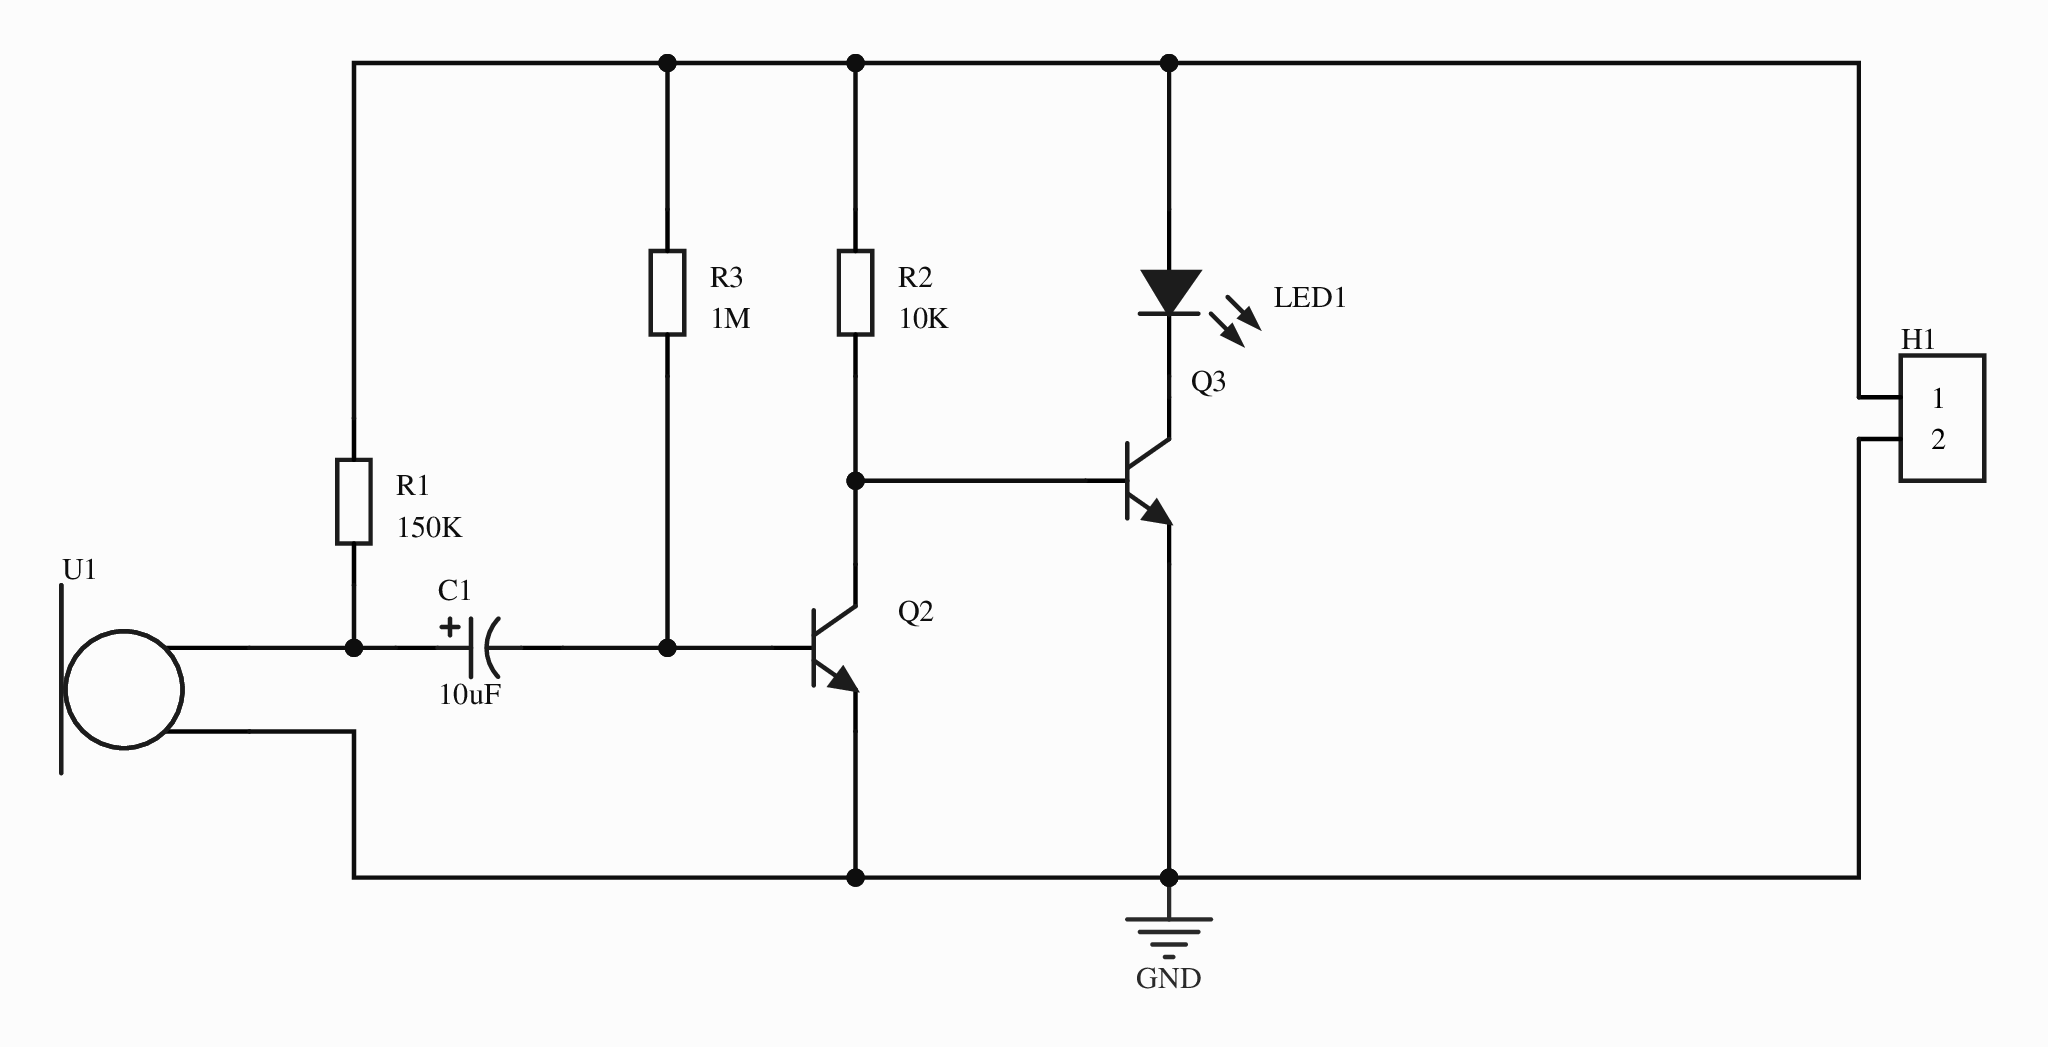
[diagram p0: MISC52075-3.schdoc]
# Altium project MISC52075-2.PrjPcb
1 sheet, 9 parts. Net scope: global (net labels, ports and power ports of the same name join across sheets).
Board file: MISC52075.pcbdoc

## Sheet MISC52075-3.schdoc
size 297 x 209 mm; Version: V1.0; @Project Name: MISC52075; @Update Date: 2026-10-05; @Create Date: 2026-10-05; @Board Name: MISC52075; @Create Time: 20:24:00; @Page Count: 1; @Page No: 1; @Schematic Name: MISC52075; @Update Time: 20:24:00; Size: A4

### Parts
C1  10uF  [CAP-TH_BD5.0-P2.00-D0.8-FD-10UF50VC110GL]
H1  (no value)  [HDR-TH_2P-P2.54-V-F]
LED1  (no value)  [LED_0603]
Q2  (no value)  [S8050_SOT-23]
Q3  (no value)  [S8050_SOT-23]
R1  150K  [R0603]
R2  10K  [R0603]
R3  1M  [R0603]
U1  电流源  [咪头]  (value not drawn)

### Nets
GND: H1.2 Q2.2 Q3.2 U1.1
NetC1_1: C1.1 R1.1 U1.2
NetC1_2: C1.2 Q2.1 R3.1
NetH1_1: H1.1 LED1.2(A) R1.2 R2.2 R3.2
NetLED1_1: LED1.1(C) Q3.3
NetQ2_3: Q2.3 Q3.1 R2.1

### Library data of the parts
C1 = 10UF50VC110GL: 容值:10uF;精度:±20%;额定电压:50V;纹波电流:120mA@100KHz;等效串联电阻(ESR):1.6Ω;; Manufacturer: Econd(米朗电子); AddInBom: yes; ModelId: b35ab6b0460c4c43a629d91cfc2b58780819f05c4eef4c71ace90d822a990e87; ModelTransform: 196.85,196.85,0,0,0,0,0,0,-196.85; Tolerance: ±20%; Voltage Rating: 50V; Equivalent Series Resistance(ESR): 1.6Ω; Pin Spacing: 2mm; Lifetime: 5000hrs@105℃; Symbol: 10UF50VC110GL; Device: 10UF50VC110GL; Value: 10uF; FootprintName: CAP-TH_BD5.0-P2.00-D0.8-FD-10UF50VC110GL; LCSC Part Name: 10uF ±20% 50V; ManufacturerPart: 10UF50VC110GL; Supplier Footprint: 插件,D5xL11mm; JLCPCB Part Class: Extended Part; Datasheet: https://item.szlcsc.com/datasheet/10UF50VC110GL/49031974.html; Supplier: LCSC; ConvertToPcb: yes; ModelName: CAP-TH_BD5.0-P2.00-D0.8-FD-10UF50VC110GL; Ripple Current: 120mA@100KHz; Diameter: 5mm; Height - Seated (Max): 11mm; Operating Temperature: -40℃~+105℃
H1 = HDR-F_2.54_1x2P: Symbol: Header-Female-2.54_1x2; ConvertToPcb: yes; ModelId: a9450ef445564560a104363b9aacde4e0819f05c4eef4c71ace90d822a990e87; ModelName: HDR-TH_2P-P2.54-F-LI-1X2P; ModelTransform: 215.7476,98.425,0,0,0,0,0,0,-129.921; Device: HDR-F_2.54_1x2P; FootprintName: HDR-TH_2P-P2.54-V-F; AddInBom: yes; SupplierPart: C49661; Supplier Footprint: 插件
LED1 = LED_0603-B: Symbol: LED_B; Convert to PCB: yes; 3D Model: eb8d964598f24248affda46f619856c50819f05c4eef4c71ace90d822a990e87; 3D Model Transform: 63.1,31.6,23.7,0,0,0,0,0,0; ModelName: LED-0603_B; Device: LED_0603-B; Add into BOM: yes; Supplier Footprint: 0603; FootprintName: LED_0603
Q2 Q3 = S8050_SOT_NPN: Symbol: NPN; 3D Model: c62791f0466c4ae2a892c056b845b0ca0819f05c4eef4c71ace90d822a990e87; 3D Model Transform: 98.6,114.12,41.29,180,0,0,0,0,-3; ConvertToPcb: yes; ModelName: SOT-23-3P_L2.9-W1.3-H1.0-LS2.4-P0.95; Device: S8050_SOT_NPN; Supplier Footprint: SOT-23; FootprintName: S8050_SOT-23; AddInBom: yes
R1 R2 = Res_0603: Symbol: 电阻; ConvertToPcb: yes; ModelId: fc143cca1e79419f9cd78b61e9279f080819f05c4eef4c71ace90d822a990e87; ModelTransform: 31.8897,63.7794,0,90,0,0,0,0,0; Device: Res_0603; FootprintName: R0603; AddInBom: yes; Supplier Footprint: 0603; ModelName: R0603
  R1: Value: 150K
  R2: Value: 10K
R3 = Res_0603: Symbol: 电阻; 3D Model: fc143cca1e79419f9cd78b61e9279f080819f05c4eef4c71ace90d822a990e87; 3D Model Transform: 31.8897,63.7794,0,90,0,0,0,0,0; ConvertToPcb: yes; Device: Res_0603; Supplier Footprint: 0603; Value: 1M; FootprintName: R0603; AddInBom: yes; ModelName: R0603
U1 = 咪头: Add into BOM: yes; Symbol: 咪头; Device: 咪头; FootprintName: 咪头; ConvertToPcb: yes